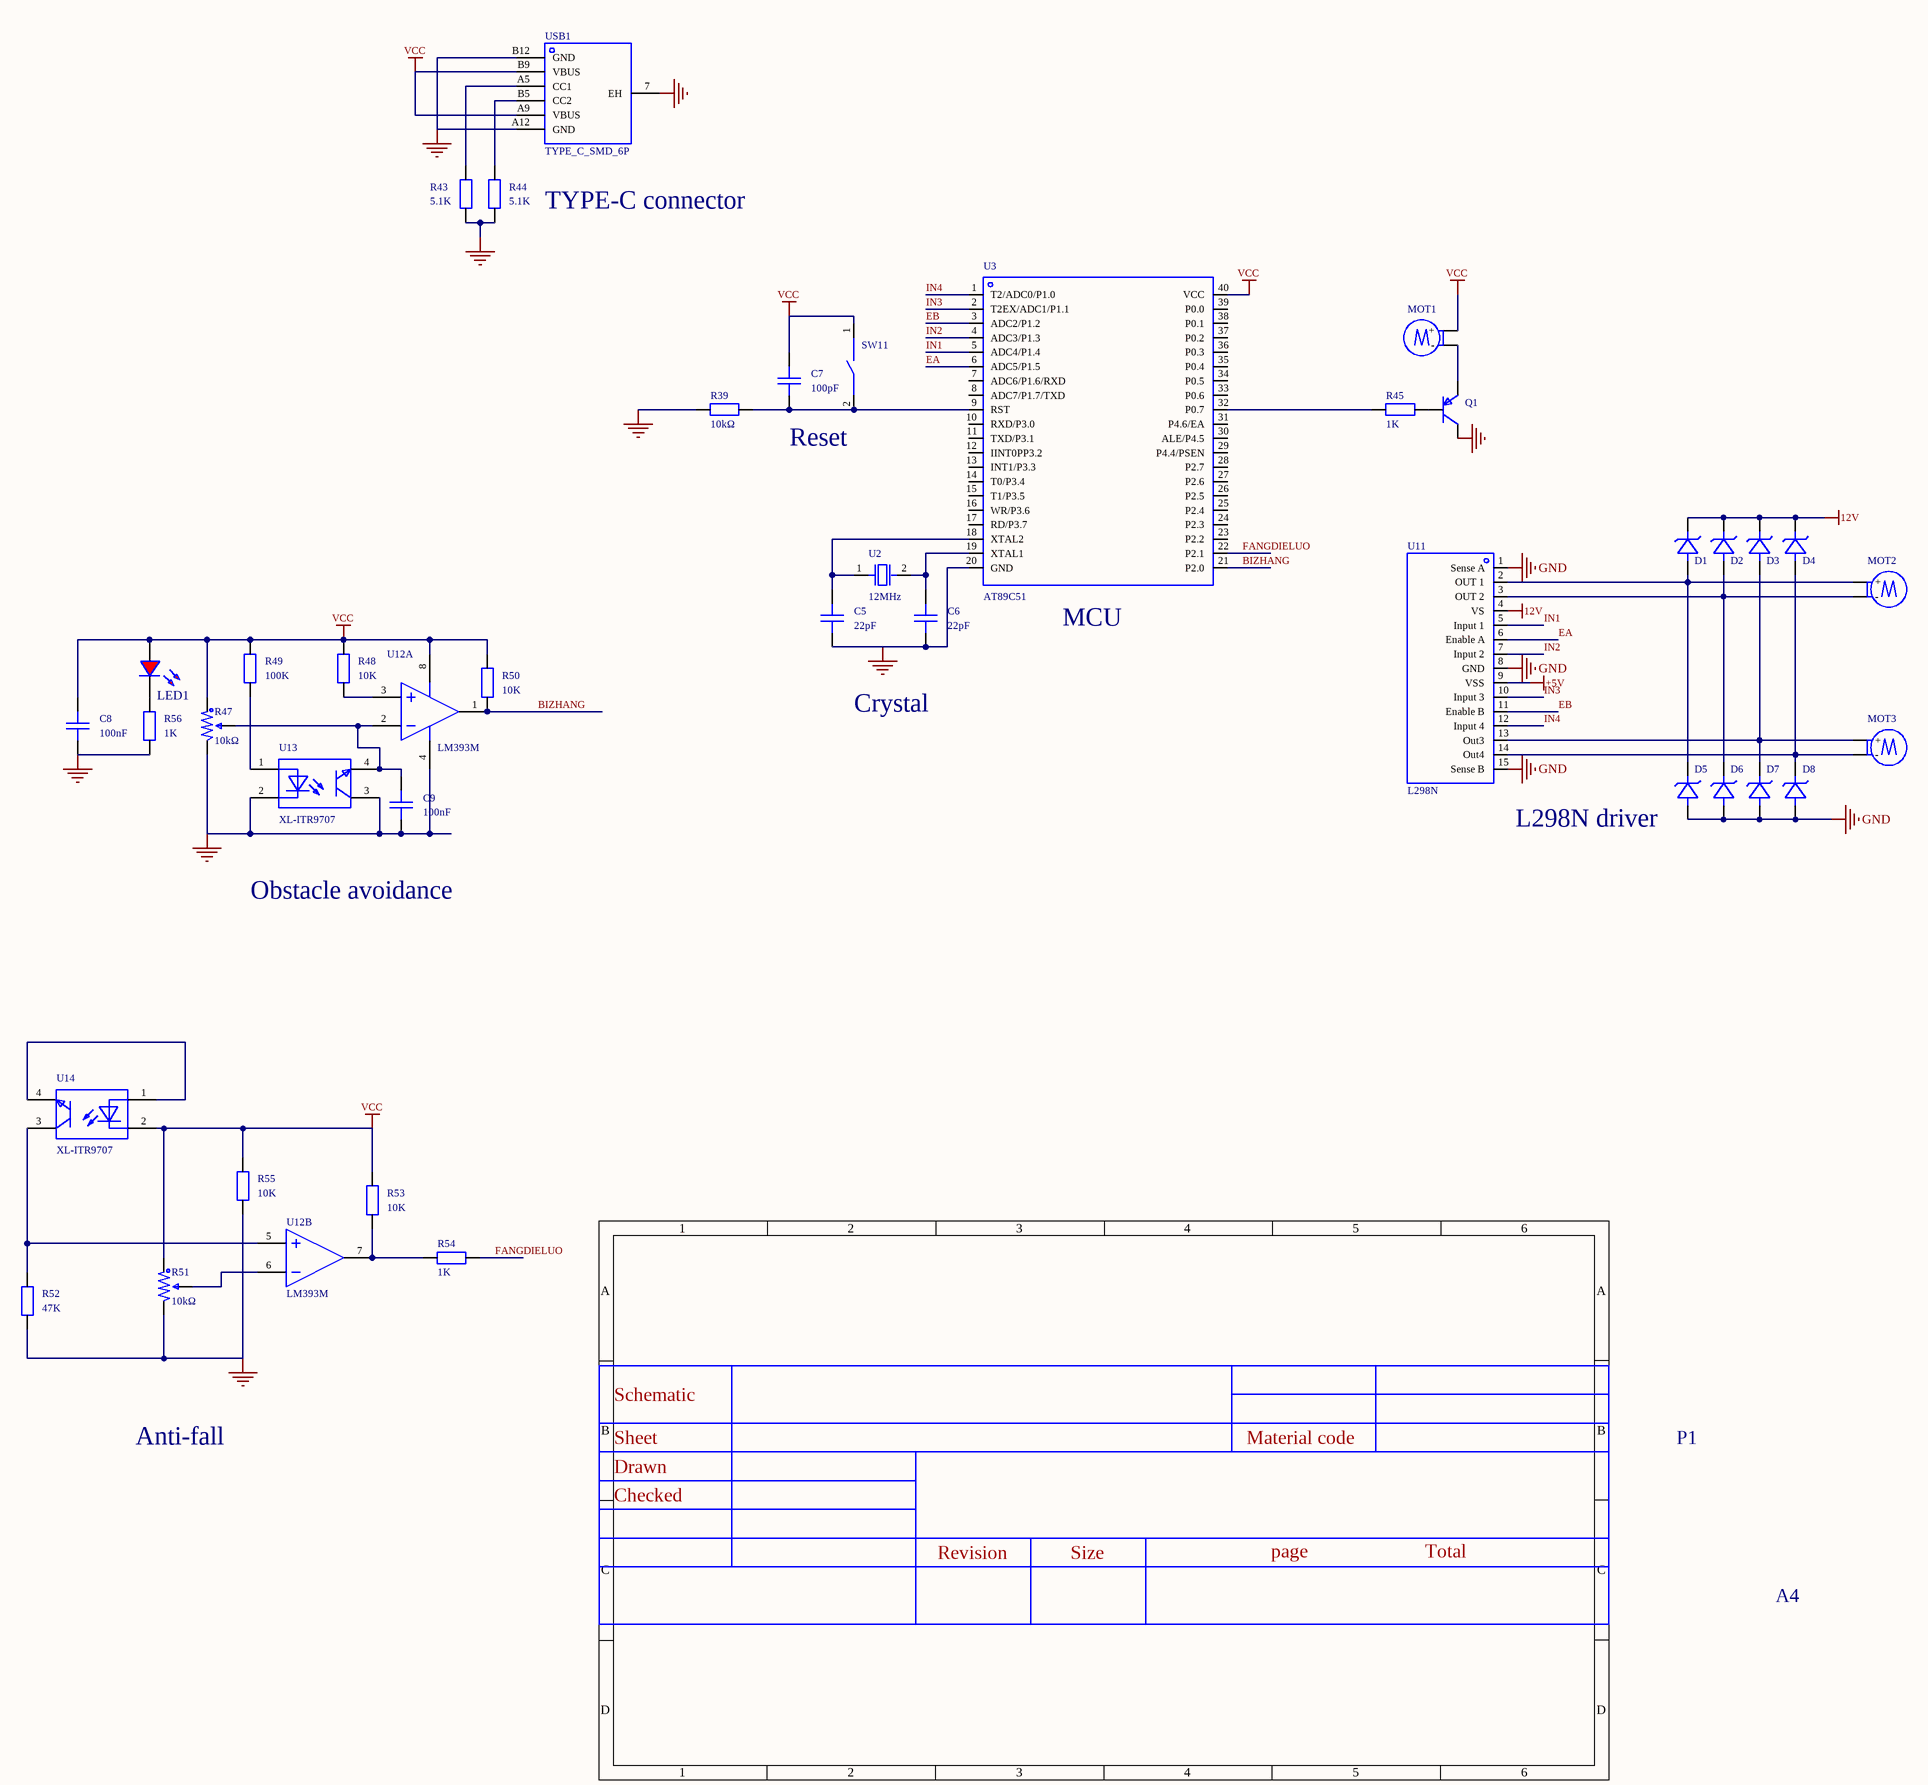
[diagram p0: MISC61231-3.schdoc]
# Altium project MISC61231-2.PrjPcb
1 sheet, 40 parts. Net scope: global (net labels, ports and power ports of the same name join across sheets).
Board file: MISC61231.pcbdoc

## Sheet MISC61231-3.schdoc
size 178 x 98 mm; Version: V1.0; @Project Name: MISC61231; @Page Count: 1; @Update Date: 2025-04-22; @Create Date: 2025-04-22; @Schematic Name: MISC61231; @Page No: 1; @Board Name: MISC61231; @Create Time: 22:50:33; @Update Time: 20:08:34

### Parts
C5  22pF  [CAP-TH_L3.6-W2.3-P5.00-D0.5]
C6  22pF  [CAP-TH_L3.6-W2.3-P5.00-D0.5]
C7  100pF  [C0603]
C8  100nF  [C0603]
C9  100nF  [C0603]
D1  (no value)  [SOD-123FL_L2.7-W1.8-LS3.8-RD]
D2  (no value)  [SOD-123FL_L2.7-W1.8-LS3.8-RD]
D3  (no value)  [SOD-123FL_L2.7-W1.8-LS3.8-RD]
D4  (no value)  [SOD-123FL_L2.7-W1.8-LS3.8-RD]
D5  (no value)  [SOD-123FL_L2.7-W1.8-LS3.8-RD]
D6  (no value)  [SOD-123FL_L2.7-W1.8-LS3.8-RD]
D7  (no value)  [SOD-123FL_L2.7-W1.8-LS3.8-RD]
D8  (no value)  [SOD-123FL_L2.7-W1.8-LS3.8-RD]
LED1  (no value)  [LED_0603]
MOT1  LCM1027A2445F  [VIBRATING-MOTOR-SMD_WELDING]  (value not drawn)
MOT2  LCM1027A2445F  [VIBRATING-MOTOR-SMD_WELDING]  (value not drawn)
MOT3  LCM1027A2445F  [VIBRATING-MOTOR-SMD_WELDING]  (value not drawn)
Q1  (no value)  [S8550P_SOT]
R39  10kΩ  [Res_1/8W]
R43  5.1K  [R0603]
R44  5.1K  [R0603]
R45  1K  [R0603]
R47  10kΩ  [RES-ADJ-SMD_RM065-V1]
R48  10K  [R0603]
R49  100K  [R0603]
R50  10K  [R0603]
R51  10kΩ  [RES-ADJ-SMD_RM065-V1]
R52  47K  [R0603]
R53  10K  [R0603]
R54  1K  [R0603]
R55  10K  [R0603]
R56  1K  [R0603]
SW11  Tactile switch, 6*6*5 plastic head, 260G, travel 0.25mm, through-hole 2-pin  [KEY-TH_2P-L6.0-W6.0-P5.00]  (value not drawn)
U2  12MHz  [HC-49US_L11.0-W4.6-P4.88]
U3  AT89C51  [DIP-40_L52.3-W13.9-P2.54-LS15.2-BL]
U11  L298N  [MULTIWATT-15_L19.6-W5.0-P1.27-L]
U12  LM393M  [SOIC-8_L4.9-W3.9-P1.27-LS6.0-BL]  (parts A,B of 2)
U13  XL-ITR9707  [OPTO-TH_4P-P2.54-XL-ITR9608]
U14  XL-ITR9707  [OPTO-TH_4P-P2.54-XL-ITR9608]
USB1  TYPE_C_SMD_6P  [TYPE-C-SMD_TYPE-C-6P]

### Nets
12V: D1.1(K) D2.1(K) D3.1(K) D4.1(K) U11.4(VS)
+5V: U11.9(VSS)
GND: C5.1 C6.1 C8.1 C9.1 D5.2(A) D6.2(A) D7.2(A) D8.2(A) Q1.3(C) R39.1 R43.1 R44.1 R47.3 R51.3 R52.1 R55.1 R56.1 U3.20(GND) U11.1(Sense_A) U11.8(GND) U11.15(Sense_B) U12.4(GND) U13.2(C) U13.3(C) USB1.7(EH) USB1.A12(GND) USB1.B12(GND)
VCC: C7.2 C8.2 LED1.2(A) MOT1.2(+) R47.1 R48.2 R49.2 R50.2 R51.1 R53.2 R55.2 SW11.1 U3.40(VCC) U12.8(VCC) U14.2(C) USB1.A9(VBUS) USB1.B9(VBUS)
BIZHANG: R50.1 U3.21(P2.0) U12.1(OUT1)
EA: U3.6(ADC5/P1.5) U11.6(Enable_A)
EB: U3.3(ADC2/P1.2) U11.11(Enable_B)
FANGDIELUO: R54.1 U3.22(P2.1)
IN1: U3.5(ADC4/P1.4) U11.5(Input_1)
IN2: U3.4(ADC3/P1.3) U11.7(Input_2)
IN3: U3.2(T2EX/ADC1/P1.1) U11.10(Input_3)
IN4: U3.1(T2/ADC0/P1.0) U11.12(Input_4)
NetC5_2: C5.2 U2.1(OSC1) U3.18(XTAL2)
NetC6_2: C6.2 U2.2(OSC2) U3.19(XTAL1)
NetC7_1: C7.1 R39.2 SW11.2 U3.9(RST)
NetC9_2: C9.2 R47.2 U12.2(IN1+) U13.4(E)
NetD1_2: D1.2(A) D5.1(K) MOT2.2(+) U11.2(OUT_1)
NetD2_2: D2.2(A) D6.1(K) MOT2.1(-) U11.3(OUT_2)
NetD3_2: D3.2(A) D7.1(K) MOT3.2(+) U11.13(Out3)
NetD4_2: D4.2(A) D8.1(K) MOT3.1(-) U11.14(Out4)
NetLED1_1: LED1.1(C) R56.2
NetMOT1_1: MOT1.1(-) Q1.2(E)
NetQ1_1: Q1.1(B) R45.2
NetR43_2: R43.2 USB1.A5(CC1)
NetR44_2: R44.2 USB1.B5(CC2)
NetR45_1: R45.1 U3.32(P0.7)
NetR48_1: R48.1 U12.3(IN1-)
NetR49_1: R49.1 U13.1(A)
NetR51_2: R51.2 U12.6(IN2-)
NetR52_2: R52.2 U12.5(IN2+) U14.3(C)
NetR53_1: R53.1 R54.2 U12.7(OUT2)
NetU14_1: U14.1(A) U14.4(E)

Not connected (* = marked no-connect by the designer): U3 7(ADC6/P1.6/RXD) 8(ADC7/P1.7/TXD) 10(RXD/P3.0) 11(TXD/P3.1) 12(IINT0PP3.2) 13(INT1/P3.3) 14(T0/P3.4) 15(T1/P3.5) 16(WR/P3.6) 17(RD/P3.7) 23(P2.2) 24(P2.3) 25(P2.4) 26(P2.5) 27(P2.6) 28(P2.7) 29(P4.4/PSEN) 30(ALE/P4.5) 31(P4.6/EA) 33(P0.6) 34(P0.5) 35(P0.4) 36(P0.3) 37(P0.2) 38(P0.1) 39(P0.0)

### Notes on the sheet
- TYPE-C connector
- Reset
- (near U3) MCU
- Crystal
- (near D5) L298N driver
- Obstacle avoidance
- Anti-fall
- 2025-04-22
- Schematic
- Sheet
- Material code
- P1
- Checked
- Drawn
- Revision
- Size
- page
- Total
- A4
- 1

### Library data of the parts
C5 C6 = K300J10C0GF5UH5: Capacitance: 30pF; tolerance: ±5%; rated voltage: 50V; temperature coefficient: C0G;; Manufacturer: VISHAY(威世); AddInBom: yes; ModelId: 8586b865f3f94c6bbd5d7f2c3c951380; ModelName: CAP-TH-2P-L3.6-W2.3-H6.2-P5.0; ModelTransform: 220.472,90.551,0,0,0,0,-0.005,0,-137.795; Value: 22pF; Symbol: K300J10C0GF5UH5; Device: K300J10C0GF5UH5; LCSC Part Name: 30pF ±5% 50V; ManufacturerPart: K300J10C0GF5UH5; Supplier Footprint: 插件; JLCPCB Part Class: Extended library; Datasheet: example.com/upload/public/pdf/source/20210702/6531D680143ED60327F22057485455BA.pdf; Supplier: LCSC; ConvertToPcb: yes; FootprintName: CAP-TH_L3.6-W2.3-P5.00-D0.5; Tolerance: ±5%; Voltage Rated: 50V; Temperature Coefficient: C0G
C7-C9 = CAP_0603: ConvertToPcb: yes; SymbolName: CapAcitance; ModelId: ac125912035d415993ca9572d50418b1; ModelName: C0603_L1.6-W0.8-H0.8; ModelTransform: 62.992,31.496,0,0,0,0,0,0,0; Device: CAP_0603; AddInBom: yes; Supplier Footprint: 0603; FootprintName: C0603
  C7: Value: 100pF
  C8 C9: Value: 100nF
D1-D8 = 1N4007: Diode configuration: single; DC reverse voltage (Vr): 1kV; average rectified current (Io): 1A; forward voltage (Vf): 1.1V@1A; reverse current (Ir): 10A@1kV;; Manufacturer: TWGMC(台湾迪嘉); Symbol: 1N4007_C727082; AddInBom: yes; ModelId: 86f9151e155e4fe2af0c4f2e0a80302e; ModelName: SOD-123FL_L2.8-W1.8-H1.1-LS3.6; ModelTransform: 141.7,70.9,0,180,0,0,0,0,0; Reverse Leakage Current: 10A@1kV; Device: 1N4007; LCSC Part Name: 1kV 1A 1.1V@1A; SupplierPart: C727082; ManufacturerPart: 1N4007; Supplier Footprint: SOD-123FL; JLCPCB Part Class: Extended Part; Datasheet: example.com/upload/public/pdf/source/20200828/C727082_2F914037E829F0E2238583225D7ED281.pdf; Supplier: LCSC; ConvertToPcb: yes; FootprintName: SOD-123FL_L2.7-W1.8-LS3.8-RD; Diode Configuration: Single; Reverse Voltage (Vr): 1kV; Average Rectified Current (Io): 1A; Forward Voltage (Vf@If): 1.1V@1A
LED1 = LED_0603-R: Symbol: LED_R; Convert to PCB: yes; 3D Model: dd8257b0d61a4cd7b68939a056e08095; 3D Model Transform: 58.72,29.4,22.03,0,0,0,0,0,0; ModelName: LED-0603_R; Device: LED_0603-R; Add into BOM: yes; Supplier Footprint: 0603; FootprintName: LED_0603
MOT1-MOT3 = LCM1027A2445F: Type: flat vibration motor; rated voltage: 3V; rated speed: 10000rpm; rotation direction: CW; CCW;; Manufacturer: LEADER(立得); AddInBom: yes; ModelId: 8f445ba560bf4287a30326e4aa2b54b1; ModelTransform: 393.5478,130.315,0,0,0,0,0,-9.843,-59.055; Rated Current: 80mA; Sense Of Rotation: CW; CCW; Symbol: LCM1027A2445F; Device: LCM1027A2445F; LCSC Part Name: 扁平1027 振动马达; SupplierPart: C2759984; ManufacturerPart: LCM1027A2445F; Supplier Footprint: -; JLCPCB Part Class: Extended library; Datasheet: example.com/upload/public/pdf/source/20210326/C2759984_5008EC97BD438BDFB6866D31635439F4.pdf; Supplier: LCSC; ConvertToPcb: yes; FootprintName: VIBRATING-MOTOR-SMD_WELDING; ModelName: VIBRATING-MOTOR-SMD_WELDING; Type: Flat vibration motor; Rated Voltage: 3V; Rated Speed: 10000rpm; Operating Temperature: -20℃~+60℃
Q1 = S8550_SOT_PNP: Symbol: PNP; ConvertToPcb: yes; ModelId: 9c0df02d6f3e44e889da37f3e5bf5496; ModelName: SOT-23-3_L2.9-W1.4-P1.90-LS2.5-BR; ModelTransform: 98.43,114.17,37.91,0,0,0,0,0,0; Device: S8550_SOT_PNP; AddInBom: yes; Supplier Footprint: SOT-23; FootprintName: S8550P_SOT
R39 = Res_AXIAL-1/8W: Symbol: Resistor; ConvertToPcb: yes; ModelId: b2b5ae7ae4c642178fe0039925c86a3f; ModelName: RES-TH_BD1.8-L3.2-P7.20-D0.4; ModelTransform: 282.86,66.88,253.09,0,0,0,0,0,-191; Device: Res_AXIAL-1/8W; AddInBom: yes; Supplier Footprint: 轴向引线; Value: 10kΩ; FootprintName: Res_1/8W
R43-R45 R48-R50 R52-R56 = Res_0603: Symbol: Resistor; ConvertToPcb: yes; ModelId: fc143cca1e79419f9cd78b61e9279f08; ModelTransform: 31.8897,63.7794,0,90,0,0,0,0,0; Device: Res_0603; AddInBom: yes; Supplier Footprint: 0603; FootprintName: R0603; ModelName: R0603
  R43 R44: Value: 5.1K
  R45 R54 R56: Value: 1K
  R48 R50 R53 R55: Value: 10K
  R49: Value: 100K
  R52: Value: 47K
R47 R51 = RM065-103(10K): Resistance: 10kΩ; tolerance: ±25%; power: 100mW;; Manufacturer: BOCHEN(博晨); AddInBom: yes; ModelId: c816c2b7942147f5a832150e8ef6960c; ModelTransform: 255.905,283.464,0,0,0,0,0.025,-3.937,-157.48; Symbol: RM065-103(10K); Device: RM065-103(10K); LCSC Part Name: 10kΩ ±25%; SupplierPart: C5205021; ManufacturerPart: RM065-103(10K); Supplier Footprint: 插件; JLCPCB Part Class: Extended Part; Datasheet: example.com/upload/public/pdf/source/20221019/6263C46FBC7F1B66CBAADA74DC5EFAA2.pdf; Supplier: LCSC; ConvertToPcb: yes; FootprintName: RES-ADJ-SMD_RM065-V1; ModelName: RES-ADJ-SMD_RM065-V1; Value: 10kΩ; Tolerance: ±25%; Power(Watts): 100mW
SW11 = 轻触开关,6*6*5塑头,260G,行程0.25mm,直插中2脚: Symbol: SWITCH,6*6*5PLASTIC HEAD,260G, 0.25MM,DIP2; AddInBom: yes; ModelId: d13ad252cbf84dc495704a853cd2bab6; ModelName: KEY-TH_2P-L6.0-W6.0-H5.0-P5.00; ModelTransform: 236.22,236.22,0,0,0,0,0,0,-137.795; Device: Tactile switch, 6*6*5 plastic head, 260G, travel 0.25mm, through-hole 2-pin; LCSC Part Name: 轻触开关,6*6*5塑头,260G,行程0.25mm,直插中2脚; SupplierPart: C71845; ManufacturerPart: 轻触开关,6*6*5塑头,260G,行程0.25mm,直插中2脚; Supplier Footprint: 插件; JLCPCB Part Class: Extended library; Supplier: LCSC; ConvertToPcb: yes; FootprintName: KEY-TH_2P-L6.0-W6.0-P5.00
U2 = ECS-120-S-4: Frequency: 12MHz; frequency tolerance at room temp: ±30ppm; external load capacitance: -; frequency stability (full temp): ±50ppm;; Manufacturer: ECS; AddInBom: yes; ModelId: 59d05c800eee432cb051aa4925461fda; ModelName: HC-49US_L11.0-W4.7-H3.5-P4.88; ModelTransform: 432.44473,183.0705,0,0,0,0,0,0,-137.795; Equivalent Series Resistance (ESR): 60Ω; Symbol: ECS-120-S-4; Device: ECS-120-S-4; LCSC Part Name: 12MHz ±30ppm; ManufacturerPart: ECS-120-S-4; Supplier Footprint: HC-49S; JLCPCB Part Class: Extended library; Datasheet: example.com/upload/public/pdf/source/20210402/81F084B668D60DFAE850A61100CCABAF.pdf; Supplier: LCSC; ConvertToPcb: yes; FootprintName: HC-49US_L11.0-W4.6-P4.88; Value: 12MHz; Normal temperature Frequency Tolerance: ±30ppm; External load capacitor: -; Frequency Stability(Full temperature range): ±50ppm; Operating Temperature: -10℃~+70℃
U3 = STC89C516RD+40I-PDIP40: CPU core: 51 series; program memory capacity: 61KB; RAM total capacity: 1.25KB; GPIO port count: 35; operating voltage range: 3.5V~5.5V; CPU max clock: -; program memory type: FLASH;; Manufacturer: STC(宏晶); AddInBom: yes; ModelId: 16d4686a009b4ddca948f91eddb57b14; ModelName: DIP-40_L52.3-W13.8-H4.0-LS15.24-P2.54; ModelTransform: 2059.051,615.743,0,0,0,0,0,0,-129.921; GPIO Ports Number: 35; 16Bit Timer: 3; UART/USART: 1; Peripheral/Function: Watchdog; Manufacturer Part: AT89C51; Symbol: STC89C516RD+40I-PDIP40; Device: STC89C516RD+40I-PDIP40; LCSC Part Name: STC89C516RD+40I-PDIP40; SupplierPart: C52225; Supplier Footprint: DIP-40; JLCPCB Part Class: Extended library; Datasheet: example.com/upload/public/pdf/source/20180614/C87831_BBAF7FB8B286C29ACE4E9B180C033FEC.pdf; Supplier: LCSC; ConvertToPcb: yes; FootprintName: DIP-40_L52.3-W13.9-P2.54-LS15.2-BL; CPU Core: 51 series; Program Storage Size: 61KB; RAM Size: 1.25KB; Operating Voltage Range: 3.5V~5.5V; CPU Maximum Speed: -; Program Memory Type: FLASH; Operating Temperature Range: -40℃~+85℃; ADC (Bit): -; DAC (Bit): -; PWM (Bit): -; 8Bit Timer: -; 32Bit Timer: -; CAN: -; I2C: -; I2S: -; SPI: -; Universal Serial Bus: -; Internal Comparator: -; communication protocol: -; Watchdog: Yes; Real-Time Clock: -; Infrared Data Association: -; Low-Voltage Detect: -; CCP Capture/Compare: -; Secure Digital Input and Output: -; Direct Memory Access: -; Internal Oscillator: -
U11 = L298N_C19922: Supply voltage: 4.5V~7V; features: overcurrent protection (OCP); overtemperature protection (OPT);; Manufacturer: ST(意法半导体); AddInBom: yes; ModelId: 17dbda3c803a45a0ac2c74e6ab5d5790; ModelTransform: 795.27392,389.3693,0,0,0,0,0,84.646,-137.795; Device: L298N_C19922; Symbol: L298N_C19922; LCSC Part Name: L298N; SupplierPart: C19922; ManufacturerPart: L298N; Supplier Footprint: Multiwatt-15-V; JLCPCB Part Class: Extended Part; Datasheet: example.com/upload/public/pdf/source/20131014/1457706655076.pdf; Supplier: LCSC; ConvertToPcb: yes; FootprintName: MULTIWATT-15_L19.6-W5.0-P1.27-L; ModelName: MULTIWATT-15_L19.6-W5.0-P1.27-L; Supply Voltage: 4.5V~7V; Feature: Overcurrent protection (OCP); overtemperature protection (OPT); Operating Temperature: -40℃~+150℃@(Tj)
U12 = LM393M_C258241: Relevance: []; AddInBom: yes; ModelId: e81d2f7d937b4a6ab1dca543ff5d56a4; ModelName: SOIC-8_L4.9-W3.9-H1.7-LS6.0-P1.27; ModelTransform: 189.751,236.22,0,0,0,0,0.0005,0.0005,0; Symbol: LM393M; Device: LM393M_C258241; LCSC Part Name: LM393M 停产; SupplierPart: C258241; ManufacturerPart: LM393M; Supplier Footprint: SOIC-8; JLCPCB Part Class: Extended library; Supplier: LCSC; ConvertToPcb: yes; FootprintName: SOIC-8_L4.9-W3.9-P1.27-LS6.0-BL
U13 U14 = XL-ITR9707: Plug-in, through-beam photoelectric switch, high reliability, high radiant intensity, low-voltage drive, fast response, high sensitivity, automatic sensor; Manufacturer: XINGLIGHT(成兴光); AddInBom: yes; ModelId: 38b0cabfeef04a988dbe53f6c2ac56c3; ModelTransform: 512.204,236.22,0,0,0,0,0.002,0,-196.85; Symbol: XL-ITR9707; Device: XL-ITR9707; LCSC Part Name: 对射式光电开关; SupplierPart: C7545635; ManufacturerPart: XL-ITR9707; Supplier Footprint: -; JLCPCB Part Class: Extended library; Datasheet: example.com/upload/public/pdf/source/20240218/073FEE17891A3A05AEDCC94F15A0269B.pdf; Supplier: LCSC; ConvertToPcb: yes; FootprintName: OPTO-TH_4P-P2.54-XL-ITR9608; ModelName: OPTO-TH_4P-P2.54-XL-ITR9608
USB1 = TYPE_C_SMD_6P: AddInBom: yes; ModelId: 3770c5585474407db939b2377e27177a; ModelName: TYPE-C-SMD_6P-L8.9-W6.8-H3.2-P1.00; ModelTransform: 351.9678,267.716,0,180,0,0,0,-48.226,-39.37; Symbol: TYPE_C_SMD_6P; Device: TYPE_C_SMD_6P; LCSC Part Name: TYPE_C_SMD_6P; SupplierPart: C9900003080; ManufacturerPart: TYPE_C_SMD_6P; Supplier Footprint: TYPE_C_USB_6P; JLCPCB Part Class: Extended library; Supplier: LCSC; ConvertToPcb: yes; FootprintName: TYPE-C-SMD_TYPE-C-6P